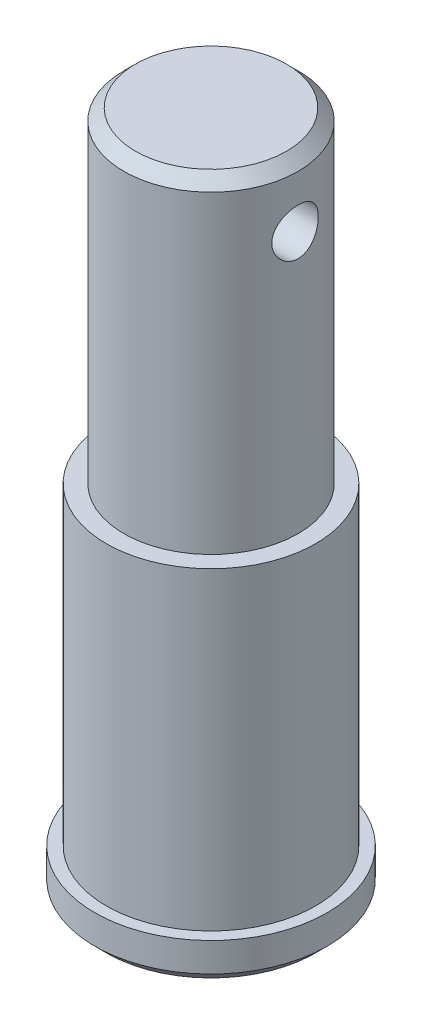
from build123d import *

# Parameters (mm, degrees)
SKETCH_2_R          = 2
CUT_EXTRUDE_1_DEPTH = 10
CHAMFER_1_SIZE      = 1


with BuildPart() as part:
    # 草图1 → 旋转1 (revolve)
    with BuildSketch(Plane.XY, mode=Mode.PRIVATE) as revolve_1_sk:
        Polygon((0, 29.25), (0, -29.25), (10, -29.25), (10, -25.75), (9, -25.75), (9, 1.25), (7.5, 1.25), (7.5, 29.25), align=None)
    revolve(revolve_1_sk.sketch.rotate(Axis((0, 29.25, 0), (0, -1, 0)), 180), axis=Axis((0, 29.25, 0), (0, -1, 0)))

    # 草图2 → 切除-拉伸1 (cut, symmetric)
    with BuildSketch(Plane(origin=(0, 0, 0), x_dir=(0, 0, -1), z_dir=(1, 0, 0))):
        with Locations((0, 23.75)):
            Circle(SKETCH_2_R)
    extrude(amount=CUT_EXTRUDE_1_DEPTH, both=True, mode=Mode.SUBTRACT)

    # 倒角1
    chamfer_1_edges = [part.edges().sort_by_distance(p)[0] for p in [
        (10, -29.25, 0),
        (7.5, 29.25, 0),
    ]]
    chamfer(chamfer_1_edges, length=CHAMFER_1_SIZE)


solid = part.part
